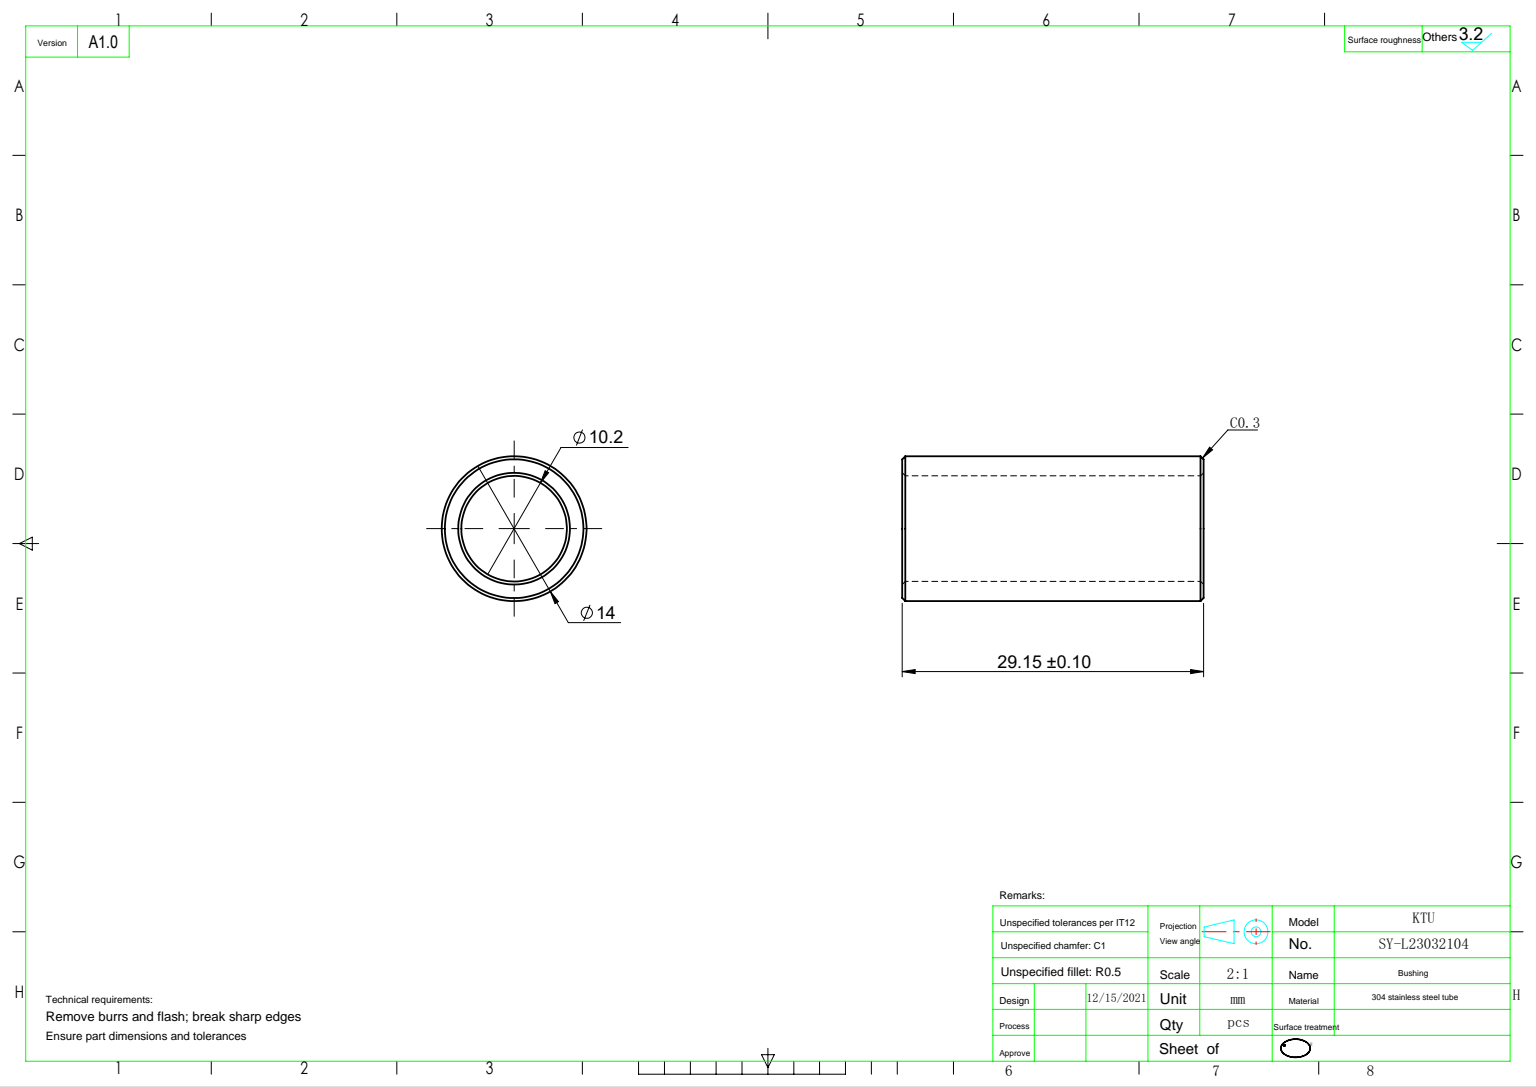
SolidWorks part; units mm, degrees
ref_plane "前视基准面" through (0, 0, 0) normal (0, 0, 1) x (1, 0, 0)
ref_plane "上视基准面" through (0, 0, 0) normal (0, 1, 0) x (1, 0, 0)
ref_plane "右视基准面" through (0, 0, 0) normal (1, 0, 0) x (0, 0, -1)
sketch "草图1" plane through (0, 0, 0) normal (0, 0, 1) x (1, 0, 0)
  circle A0 centre (0, 0) radius 7
  circle A1 centre (0, 0) radius 5.1
  dimension "D1" = 10.2
  dimension "D2" = 14
extrude "凸台-拉伸1" add sketch "草图1" along normal blind 29.15
chamfer "倒角1" distance 0.3 angle 45 1 edges at (7, 0, 0)
chamfer "倒角2" distance 0.3 angle 45 3 edges at (5.1, 0, 0) (5.1, 0, 29.15) (7, 0, 29.15)
